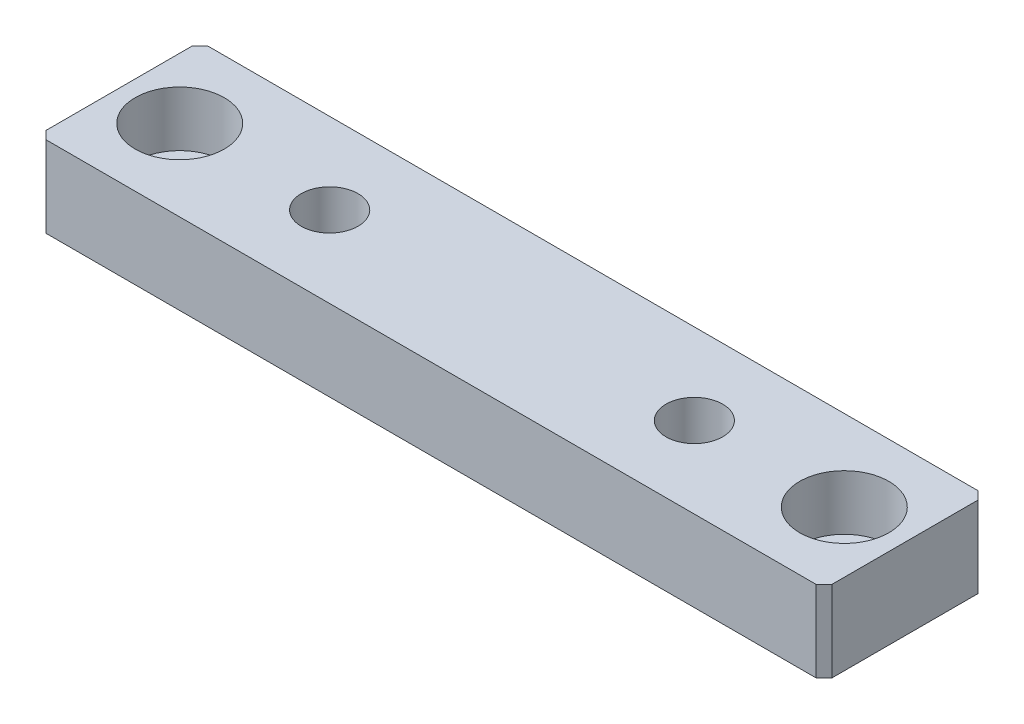
SolidWorks part; units mm, degrees
material "45#"
ref_plane "前基準面" through (0, 0, 0) normal (0, 0, 1) x (1, 0, 0)
ref_plane "上基準面" through (0, 0, 0) normal (0, 1, 0) x (1, 0, 0)
ref_plane "右基準面" through (0, 0, 0) normal (1, 0, 0) x (0, 0, -1)
sketch "草图1" plane through (0, 0, 0) normal (0, 1, 0) x (1, 0, 0)
  line L1 (-48.5, -10) -> (48.5, -10)
  line L2 (-48.5, -10) -> (-48.5, 10)
  line L3 (-48.5, 10) -> (48.5, 10)
  line L4 (48.5, -10) -> (48.5, 10)
  line L5 (-48.5, -10) -> (48.5, 10) construction
  line L6 (-48.5, 10) -> (48.5, -10) construction
  point P0 (0, 0)
  dimension "D1" = 97
  dimension "D2" = 20
extrude "凸台-拉伸1" add sketch "草图1" along normal mid plane 10
sketch "草图7" plane through (0, -5, 0) normal (0, -1, 0) x (1, 0, 0)
  line L0 (-48.5, 10) -> (48.5, 10) construction
  line L1 (48.5, -10) -> (33.5, -10)
  line L2 (48.5, -10) -> (48.5, 10)
  line L3 (48.5, 10) -> (33.5, 10)
  line L4 (33.5, -10) -> (33.5, 10)
  line L5 (0, -16.6884) -> (0, 0) construction
  line L6 (-33.5, -10) -> (-33.5, 10)
  line L7 (-48.5, 10) -> (-33.5, 10)
  line L8 (-48.5, -10) -> (-48.5, 10)
  line L9 (-48.5, -10) -> (-33.5, -10)
  dimension "D1" = 15
extrude "凸台-拉伸2" [suppressed] add sketch "草图7" along normal blind 5
hole_wizard "M8x1.0 螺纹孔1" positions "草图3" profile "草图4" tap size "M8x1.0" standard "GB" end condition through all
sketch "草图3" plane through (0, 5, 0) normal (0, 1, 0) x (1, 0, 0)
  line L0 (0, 0) -> (0, -17.7345) construction
  line L2 (0, 0) -> (-57.0299, 0) construction
  point P0 (-22.5, 0)
  point P17 (22.5, 0)
  dimension "D1" = 45
sketch "草图4" plane through (-22.5, 5, 0) normal (1, 0, 0) x (0, 0, 1)
  line L0 (0, 0) -> (0, 10)
  line L1 (0, 10) -> (3.5, 10)
  line L2 (3.5, 10) -> (3.5, 0)
  line L5 (3.5, 0) -> (0, 0)
  line L11 (0, -6.35) -> (0, 107.95) construction
  dimension "通孔螺纹孔钻头直径" = 7
  dimension "通孔螺纹孔钻头深度" = 10
cosmetic thread "孔螺蚊线1"
cosmetic thread "孔螺蚊线2"
hole_wizard "M6 六角圆柱头螺钉的柱形沉头孔1" positions "草图5" profile "草图6" counterbore size "M6" standard "GB" end condition through all
sketch "草图5" plane through (0, 5, -3) normal (0, 1, 0) x (-1, 0, 0)
  line L6 (41, -7) -> (41, 30.7238) construction
  line L7 (-48.5, -7) -> (48.5, -7) construction
  line L13 (0, -7) -> (0, 19.6401) construction
  line L15 (48.5, 3) -> (-53.805, 3) construction
  line L16 (48.5, -7) -> (48.5, 13) construction
  point P0 (41, 3)
  point P11 (-41, 3)
  dimension "D1" = 7.5
sketch "草图6" plane through (-41, 5, 0) normal (1, 0, 0) x (0, 0, 1)
  line L0 (0, 0) -> (0, 10)
  line L1 (0, 10) -> (3.3, 10)
  line L3 (3.3, 10) -> (3.3, 6.8)
  line L4 (3.3, 6.8) -> (5.5, 6.8)
  line L5 (5.5, 6.8) -> (5.5, 0)
  line L7 (5.5, 0) -> (0, 0)
  line L11 (0, -6.35) -> (0, 107.95) construction
  dimension "通孔孔直径" = 6.6
  dimension "通孔孔深度" = 10
  dimension "柱形沉头孔直径" = 11
  dimension "柱形沉头孔深度" = 6.8
chamfer "倒角1" distance 1 angle 45 4 edges at (-48.5, 0, -10) (48.5, 0, -10) (48.5, 0, 10) (-48.5, 0, 10)
